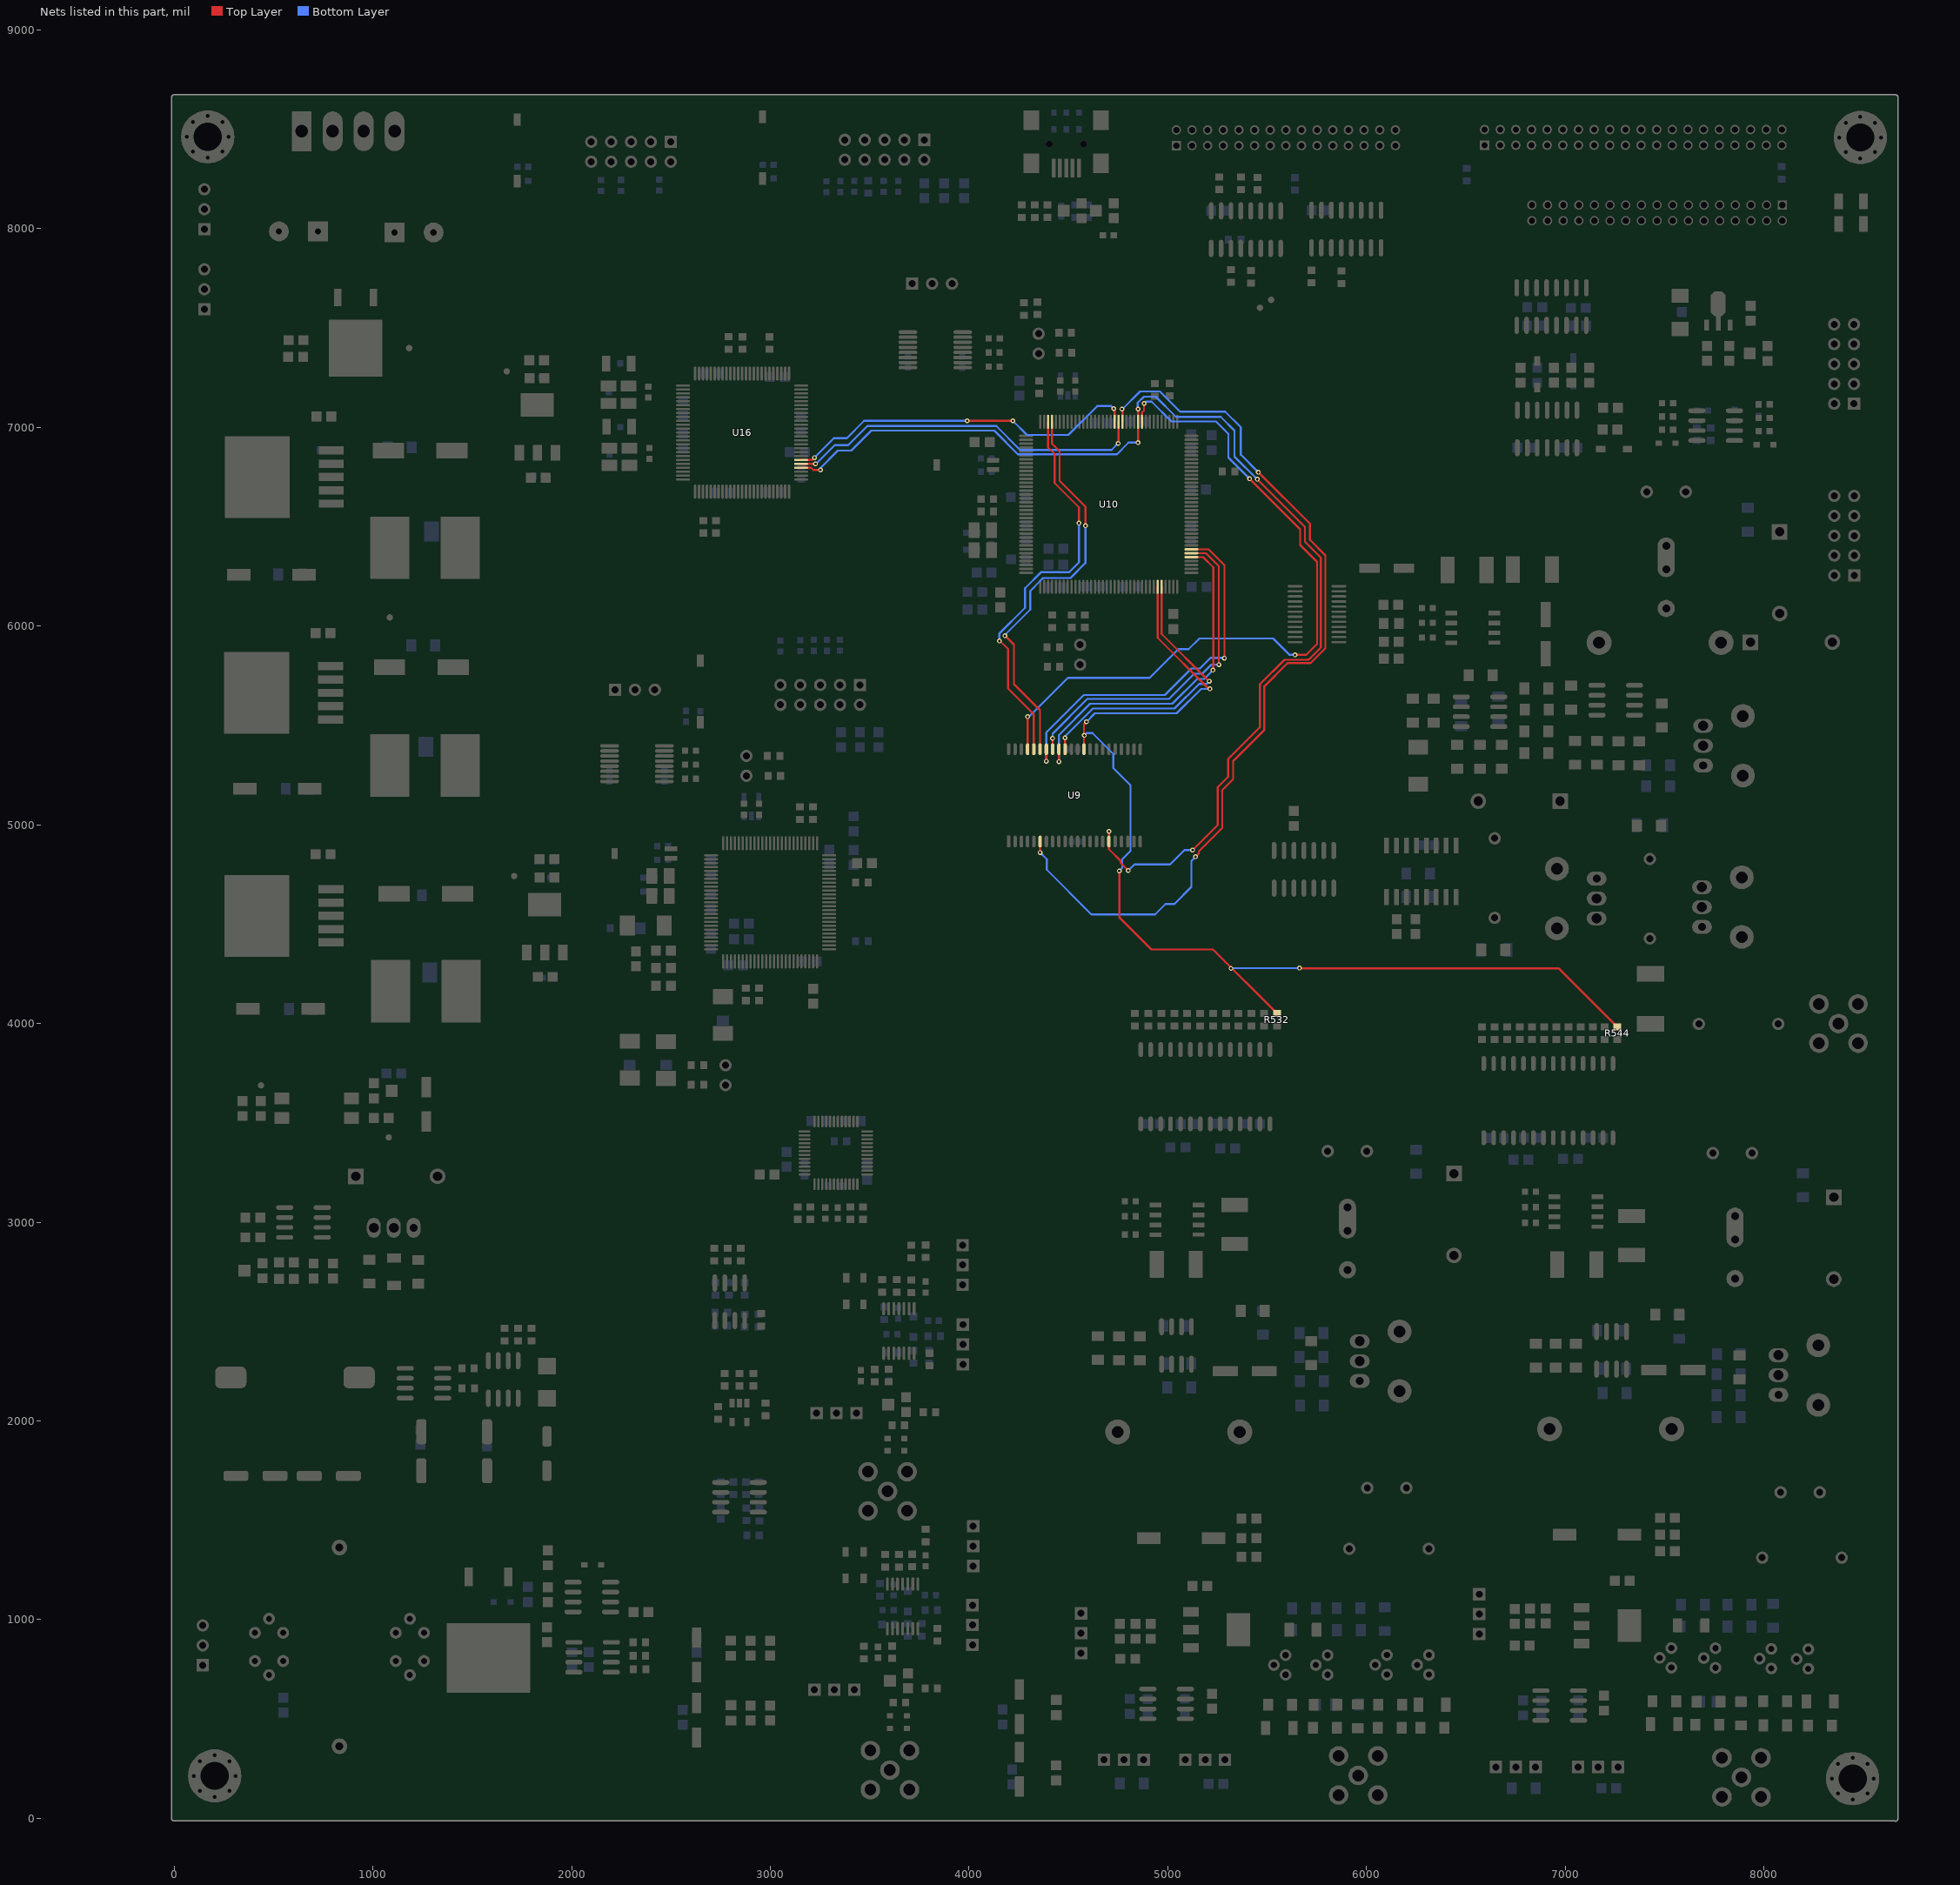
[diagram p0: the nets of this part, all layers, seen from the top]
# Altium PCB MISC82309.PcbDoc (part 7 of 14)
Units mil, origin at the board's own origin, x right, y up, seen from the top; angles counter-clockwise.
Board outline 8687.03 x 8687.86 mil, 4 copper layers (Top Layer, GND, POWER, Bottom Layer); 747 components, 583 nets, 2530 pads, 1834 vias.

## Via types
v1: diameter 24, hole 12, Top Layer to Bottom Layer, 1799 vias
v2: diameter 30, hole 15, Top Layer to Bottom Layer, 26 vias
v3: diameter 40, hole 20, Top Layer to Bottom Layer, 9 vias

## Nets (pads, with @x,y where several pads share a name; then routed paths per layer and width w, separated by ;. In a path a pad name is that pad's centre, name@x,y a point inside that pad or via, vN(x,y) a via of type N, cw(c..) or ccw(c..) an arc to the next point about the centre after c; other vN are vias at no path point) (continued)
FSMC_D11: R532.2 R544.2 U9.32 U10.67 | length 5596.7
  Top Layer w10: U9.32@4577.95,5380.57 4577.95,5505.95 v1(4591,5519) ; v1(4756,4768) 4756,4535 4918,4373 5227,4373 5549.5,4050.5 R532.2@5550,4050.5 ; U10.67@4949.06,6197.65 4949.06,5940.94 5206,5684 v1(5212,5684) ; v1(5663,4279) v1@5664,4278 ; v1@5664,4275 5666,4277 6968,4277 R544.2@7262,3983
  Bottom Layer w10: v1(4580,5450) 4592,5462 4621,5462 4726,5357 4726,5285 4812,5199 4812,4868 4771,4827 4771,4783 v1(4756,4768) ; v1(4591,5519) 4633,5561 5045,5561 5168,5684 v1(5212,5684) ; v1(5318,4278) 5319,4279 v1(5663,4279)
FSMC_D12: U9.35 U10.68 | length 1481.3
  Top Layer w10: U9.35@4483.47,5380.57 v1(4483.47,5437.47) ; U10.68@4968.75,6197.65 4968.75,5960.25 5206,5723 v1(5209,5723)
  Bottom Layer w10: v1(4483.47,5437.47) 4483.47,5445.47 4623,5585 5034,5585 5158,5709 5195,5709 v1(5209,5723)
FSMC_D13: U9.36 U10.77 | length 1756.4
  Top Layer w10: v1(4451.97,5318.03) U9.36@4451.97,5380.57 ; U10.77@5118.35,6347.25 5177.75,6347.25 5229,6296 v1@5229,5778
  Bottom Layer w10: v1(4451.97,5318.03) 4451.97,5451.97 4609,5609 5023,5609 5148,5734 5183,5734 v1(5227,5778)
FSMC_D14: U9.37 U10.78 | length 1719.9
  Top Layer w10: U9.37@4420.47,5380.57 v1(4420.47,5435.47) ; U10.78@5118.35,6366.94 5192.06,6366.94 5257,6302 v1(5257,5806)
  Bottom Layer w10: v1(4420.47,5435.47) 4420.47,5458.47 4595,5633 5006,5633 5133,5760 5173,5760 5219,5806 v1(5257,5806)
FSMC_D15: U9.38 U10.79 | length 1923.5
  Top Layer w10: v1(4388.98,5320.02) U9.38@4388.98,5380.57 ; U10.79@5118.35,6386.62 5205.38,6386.62 5285,6307 v1(5285,5839)
  Bottom Layer w10: v1(4388.98,5320.02) 4388.98,5464.98 4577,5653 4985,5653 5119,5787 5162,5787 5215,5840 v1@5284,5840
FSMC_NBL0: U9.39 U10.141 | length 2038.2
  Top Layer w10: v1@4182,5951 4226,5907 4226,5708 4357.48,5576.52 U9.39@4357.48,5380.57 ; U10.141@4417.57,7028.35 4417.57,6918.43 4456,6880 4456,6731 4586,6601 v1(4586,6505)
  Bottom Layer w10: v1@4179,5952 4179,5954 4308,6083 4308,6176.47 4358.76,6227.24 ; 4358,6228 4372,6242 4510,6242 4586,6318 v1(4586,6505)
  other v1: 4180,5951
FSMC_NBL1: U9.40 U10.142 | length 2033.3
  Top Layer w10: v1(4152,5925) v1@4152,5926 ; v1@4155,5926 4196,5885 4196,5686 4325.98,5556.02 U9.40@4325.98,5380.57 ; U10.142@4397.88,7028.35 4397.88,6900.12 4431,6867 4431,6720 4553,6598 v1(4553,6518)
  Bottom Layer w10: v1(4152,5925) 4152,5962 4282,6092 4282,6190 4364,6272 4504.47,6272 4553,6320.52 v1(4553,6518)
FSMC_NE1: U9.6 U10.123 | length 4651.4
  Top Layer w10: v1(4357.48,4860.48) U9.6@4357.48,4916 ; v1(4769,7092) 4772,7092 4771.9,7091.9 U10.123@4771.9,7028.35 ; v1(5140,4839) 5156,4855 5156,4866 5274,4984 5274,5175 5329,5230 5329,5321 5486,5478 5486,5697 5602.81,5813.81 5710.83,5813.81 5711.02,5814 5719,5814 5793,5888 5793,6356 5715,6434 5715,6515 v1(5455.73,6774.27) v1@5457.73,6774.27
  Bottom Layer w10: v1(4357.48,4860.48) 4391,4826.96 4391,4774 4616,4549 4936,4549 4989,4602 5033,4602 5119,4688 5119,4818 v1(5140,4839) ; v1(4769,7092) 4772,7092 4861,7181 4960,7181 5062,7079 5289,7079 5367,7001 5367,6863 v1(5455.73,6774.27) v1@5457.73,6774.27
FSMC_NE2: U10.124 U16.55 | length 1842.1
  Top Layer w10: U16.55@3155.24,6816.52 v1(3227.52,6816.52) ; v1@4750,6922 4752,6924 4752,7028.14 U10.124@4752.21,7028.35
  Bottom Layer w10: v1(3227.52,6816.52) 3229.52,6816.52 3324,6911 3392,6911 3488,7007 4137,7007 4257,6887 4717,6887 v1@4747,6917 ; v1@4751,6917 v1(4751,6919)
FSMC_NE3: U10.125 U16.56 | length 1818.2
  Top Layer w10: U16.56@3155.24,6836.2 3210.2,6836.2 v1(3222,6848) ; v1(3991,7033) v1(4220,7033) ; v1(4728,7094) 4730,7094 4733,7091 4732.53,7090.53 U10.125@4732.53,7028.35
  Bottom Layer w10: v1(3222,6848) 3320,6946 3385,6946 3472,7033 v1(3991,7033) ; v1(4220,7033) 4291,6962 4500,6962 4645,7107 4715,7107 v1(4728,7094)
FSMC_NOE: U9.41 U10.118 | length 3685.7
  Top Layer w10: U9.41@4294.49,5380.57 4294.49,5433.49 ; 4295,5434 v1(4295,5544) ; U10.118@4870.32,7028.35 4870.32,7074.32 4880,7084 v1@4880,7121 ; v1(5412,6741) 5666,6487 5666,6408 5751,6323 5751,5910 5696,5855 v1(5640,5855) v1@5640,5850
  Bottom Layer w10: v1@4301,5544 4497,5740 4909,5740 5053,5884 5105,5884 5159,5938 5530,5938 5613,5855 v1@5635,5855 ; v1@4880,7121 v1(4881,7121) 4889,7129 4919,7129 5018,7030 5243,7030 5305,6968 5305,6848 v1(5412,6741) ; v1@5641,5855 v1(5640,5855) ; v1@5635,5855 v1(5640,5855) ; v1@5635,5855 5637.5,5852.5 5640,5850 v1(5640,5855)
FSMC_NWE: U9.17 U10.119 U16.54 | length 5855
  Top Layer w10: U16.54@3155.24,6796.83 3205.21,6796.83 3216.04,6786 v1(3252,6786) ; v1(4703.94,4966.94) U9.17@4703.94,4916 4703.94,4877.06 4762,4819 4762,4809 v1(4801,4770) ; v1@4850,6926 4850.64,6926.64 U10.119@4850.64,7028.35 4850.64,7091.64 v1(4851,7092) ; v1(5125,4873) 5251,4999 5251,5189 5304,5242 5304,5331 5464,5491 5464,5708 5586.81,5830.81 5703.79,5830.81 5703.98,5831 5709,5831 5770,5892 5770,6345 5690,6425 5690,6499 v1(5450,6739)
  Bottom Layer w10: v1@3252,6795 3340,6883 3407,6883 3508,6984 4127,6984 4247,6864 4743,6864 4803,6924 v1@4849,6924 ; v1(4801,4770) 4832,4801 5012,4801 5084,4873 v1(5125,4873) ; v1(4851,7092) 4848,7095 4848,7123 4880,7155 4939,7155 5041,7053 5267,7053 5336,6984 5336,6853 v1(5450,6739)
  other v1: 4850,6923